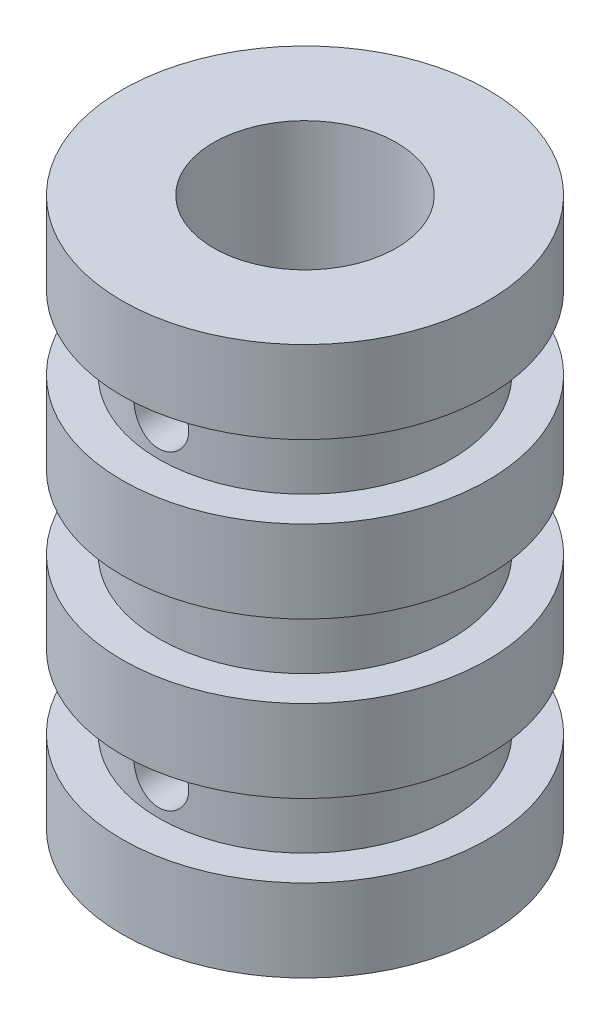
SolidWorks part; units mm, degrees
material "Plain Carbon Steel"
ref_plane "Front Plane" through (0, 0, 0) normal (0, 0, 1) x (1, 0, 0)
ref_plane "Top Plane" through (0, 0, 0) normal (0, 1, 0) x (1, 0, 0)
ref_plane "Right Plane" through (0, 0, 0) normal (1, 0, 0) x (0, 0, -1)
sketch "Sketch1" plane through (0, 0, 0) normal (0, 0, 1) x (1, 0, 0)
  line L0 (0, 0) -> (0, 30) construction
  line L1 (2.5, 15) -> (2.5, 0)
  line L2 (2.5, 0) -> (10, 0)
  line L3 (10, 0) -> (10, 4.5)
  line L4 (10, 30) -> (5, 30)
  line L5 (2.5, 15) -> (5, 15)
  line L6 (5, 15) -> (5, 30)
  line L9 (10, 25.5) -> (10, 30)
  line L10 (10, 25.5) -> (8, 25.5)
  line L11 (10, 21.5) -> (8, 21.5)
  line L12 (8, 25.5) -> (8, 21.5)
  line L13 (10, 17) -> (10, 21.5)
  line L14 (10, 17) -> (8, 17)
  line L15 (10, 13) -> (8, 13)
  line L16 (8, 17) -> (8, 13)
  line L17 (10, 8.5) -> (10, 13)
  line L18 (10, 8.5) -> (8, 8.5)
  line L19 (10, 4.5) -> (8, 4.5)
  line L20 (8, 8.5) -> (8, 4.5)
  dimension "D1" = 30
  dimension "D2" = 20
  dimension "D3" = 5
  dimension "D4" = 2
  dimension "D5" = 4
  dimension "D6" = 10
  dimension "D7" = 15
revolve "Revolve1" add sketch "Sketch1" angle 360 about L0
sketch "Sketch2" plane through (0, 0, 0) normal (0, 0, 1) x (1, 0, 0)
  line L0 (-8, 8.5) -> (8, 8.5) construction
  line L1 (-8, 25.5) -> (8, 25.5) construction
  circle A0 centre (0, 23.5) radius 1.5
  circle A1 centre (0, 6.5) radius 1.5
  dimension "D1" = 2
  dimension "D2" = 2
  dimension "D3" = 3
extrude "Cut-Extrude1" cut sketch "Sketch2" along normal up to next
